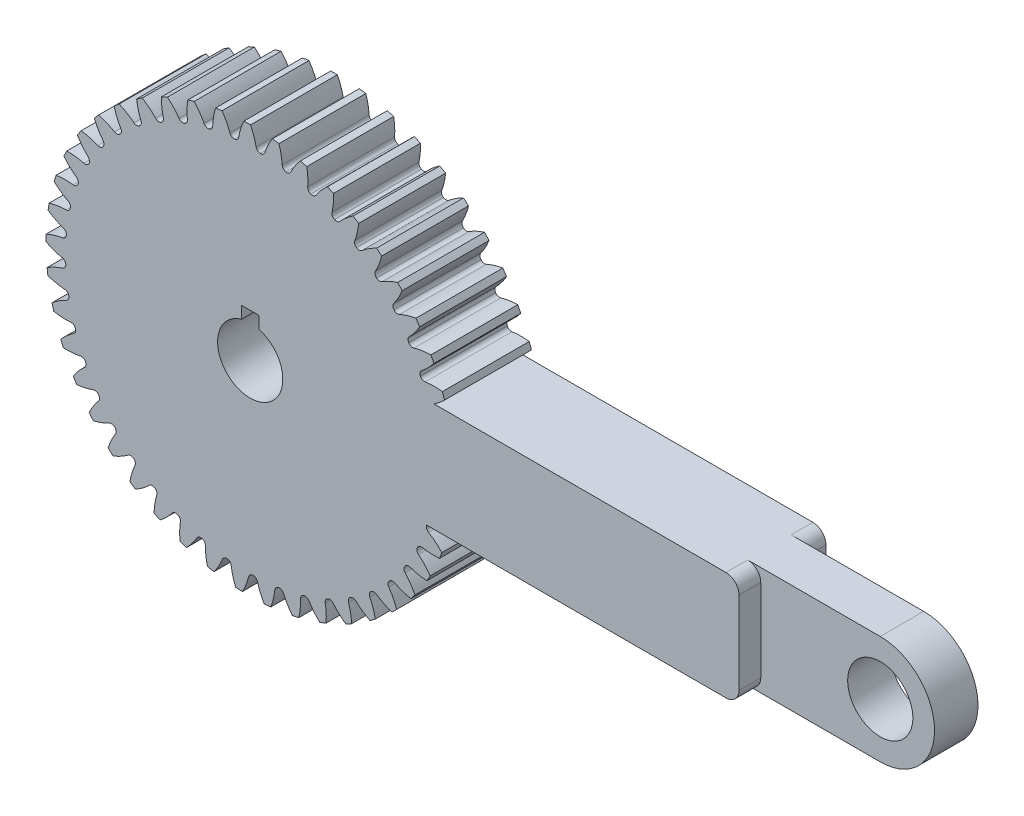
SolidWorks part; units mm, degrees
ref_plane "Front Plane" through (0, 0, 0) normal (0, 0, 1) x (1, 0, 0)
ref_plane "Top Plane" through (0, 0, 0) normal (0, 1, 0) x (1, 0, 0)
ref_plane "Right Plane" through (0, 0, 0) normal (1, 0, 0) x (0, 0, -1)
ref_plane "Plane1" through (0, 0, 0) normal (0, 0, -1) x (-1, 0, 0)
sketch "Sketch1" plane through (0, 0, 0) normal (0, 0, -1) x (-1, 0, 0)
  line L0 (-2, 7.2284) -> (-2, 10)
  line L1 (-2, 10) -> (2, 10)
  line L2 (2, 10) -> (2, 7.2284)
  line L3 (-140, -12.5) -> (-40.6202, -12.5)
  line L4 (-42.285, 12.5) -> (-140, 12.5)
  arc A0 (2, 7.2284) -> (-2, 7.2284) centre (0, 0) cw
  arc A1 (-140, 12.5) -> (-140, -12.5) centre (-140, 0) ccw
  arc A2 (-40.6202, -12.5) -> (-40.6, -12.5654) centre (0, 0) ccw
  arc A3 (-40.6, -12.5654) -> (-41.0442, -13.7206) centre (-41.5553, -12.8611) cw
  arc A4 (-44.1067, -16.2358) -> (-41.0442, -13.7206) centre (-33.1834, -26.4137) cw
  arc A5 (-44.1067, -16.2358) -> (-43.552, -17.6699) centre (0, 0) ccw
  arc A6 (-39.5941, -17.4696) -> (-43.552, -17.6699) centre (-42.3312, -2.5814) cw
  arc A7 (-39.5941, -17.4696) -> (-38.4882, -18.0253) centre (-39.3938, -18.4494) cw
  arc A8 (-38.4882, -18.0253) -> (-38.4561, -18.0936) centre (0, 0) ccw
  arc A9 (-38.4561, -18.0936) -> (-38.7352, -19.2993) centre (-39.361, -18.5193) cw
  arc A10 (-41.4178, -22.2163) -> (-38.7352, -19.2993) centre (-29.1844, -30.7749) cw
  arc A11 (-41.4178, -22.2163) -> (-40.669, -23.5592) centre (0, 0) ccw
  arc A12 (-36.7775, -22.8101) -> (-40.669, -23.5592) centre (-41.56, -8.4477) cw
  arc A13 (-36.7775, -22.8101) -> (-35.605, -23.2064) centre (-36.4428, -23.7524) cw
  arc A14 (-35.605, -23.2064) -> (-35.5637, -23.2695) centre (0, 0) ccw
  arc A15 (-35.5637, -23.2695) -> (-35.6723, -24.5024) centre (-36.4005, -23.817) cw
  arc A16 (-37.9229, -27.7643) -> (-35.6723, -24.5024) centre (-24.6174, -34.5371) cw
  arc A17 (-37.9229, -27.7643) -> (-36.9944, -28.9899) centre (0, 0) ccw
  arc A18 (-33.245, -27.7065) -> (-36.9944, -28.9899) centre (-39.9799, -14.1495) cw
  arc A19 (-33.245, -27.7065) -> (-32.0288, -27.9358) centre (-32.7824, -28.5931) cw
  arc A20 (-32.0288, -27.9358) -> (-31.9791, -27.9926) centre (0, 0) ccw
  arc A21 (-31.9791, -27.9926) -> (-31.9151, -29.2286) centre (-32.7316, -28.6512) cw
  arc A22 (-33.6898, -32.7719) -> (-31.9151, -29.2286) centre (-19.5712, -37.6271) cw
  arc A23 (-33.6898, -32.7719) -> (-32.5997, -33.8564) centre (0, 0) ccw
  arc A24 (-29.0655, -32.0637) -> (-32.5997, -33.8564) centre (-37.6216, -19.5759) cw
  arc A25 (-29.0655, -32.0637) -> (-27.8292, -32.1214) centre (-28.484, -32.8772) cw
  arc A26 (-27.8292, -32.1214) -> (-27.7721, -32.1708) centre (0, 0) ccw
  arc A27 (-27.7721, -32.1708) -> (-27.5366, -33.3858) centre (-28.4256, -32.9278) cw
  arc A28 (-28.8009, -37.1417) -> (-27.5366, -33.3858) centre (-14.144, -39.9847) cw
  arc A29 (-28.8009, -37.1417) -> (-27.5706, -38.0639) centre (0, 0) ccw
  arc A30 (-24.3202, -35.7968) -> (-27.5706, -38.0639) centre (-34.531, -24.6213) cw
  arc A31 (-24.3202, -35.7968) -> (-23.0879, -35.6819) centre (-23.6311, -36.5215) cw
  arc A32 (-23.0879, -35.6819) -> (-23.0245, -35.7228) centre (0, 0) ccw
  arc A33 (-23.0245, -35.7228) -> (-22.6223, -36.8933) centre (-23.5663, -36.5634) cw
  arc A34 (-23.3515, -40.7886) -> (-22.6223, -36.8933) centre (-8.4416, -41.564) cw
  arc A35 (-23.3515, -40.7886) -> (-22.0048, -41.5306) centre (0, 0) ccw
  arc A36 (-19.1016, -38.8331) -> (-22.0048, -41.5306) centre (-30.7683, -29.1875) cw
  arc A37 (-19.1016, -38.8331) -> (-17.8972, -38.5479) centre (-18.3184, -39.4549) cw
  arc A38 (-17.8972, -38.5479) -> (-17.8288, -38.5796) centre (0, 0) ccw
  arc A39 (-17.8288, -38.5796) -> (-17.2675, -39.6826) centre (-18.2483, -39.4873) cw
  arc A40 (-17.4476, -43.6415) -> (-17.2675, -39.6826) centre (-2.5748, -42.3343) cw
  arc A41 (-17.4476, -43.6415) -> (-16.0107, -44.1889) centre (0, 0) ccw
  arc A42 (-13.5111, -41.1136) -> (-16.0107, -44.1889) centre (-26.4068, -33.1856) cw
  arc A43 (-13.5111, -41.1136) -> (-12.3582, -40.6635) centre (-12.649, -41.6203) cw
  arc A44 (-12.3582, -40.6635) -> (-12.286, -40.6854) centre (0, 0) ccw
  arc A45 (-12.286, -40.6854) -> (-11.5767, -41.6996) centre (-12.5751, -41.6427) cw
  arc A46 (-11.2041, -45.645) -> (-11.5767, -41.6996) centre (3.342, -42.2807) cw
  arc A47 (-11.2041, -45.645) -> (-9.705, -45.9871) centre (0, 0) ccw
  arc A48 (-7.6577, -42.5939) -> (-9.705, -45.9871) centre (-21.5312, -36.5377) cw
  arc A49 (-7.6577, -42.5939) -> (-6.5787, -41.9877) centre (-6.7335, -42.9757) cw
  arc A50 (-6.5787, -41.9877) -> (-6.5042, -41.9994) centre (0, 0) ccw
  arc A51 (-6.5042, -41.9994) -> (-5.6606, -42.905) centre (-6.6572, -42.9876) cw
  arc A52 (-4.7425, -46.7601) -> (-5.6606, -42.905) centre (9.1938, -41.4041) cw
  arc A53 (-4.7425, -46.7601) -> (-3.2104, -46.8902) centre (0, 0) ccw
  arc A54 (-1.6553, -43.2451) -> (-3.2104, -46.8902) centre (-16.2366, -39.1787) cw
  arc A55 (-1.6553, -43.2451) -> (-0.6711, -42.4947) centre (-0.6869, -43.4946) cw
  arc A56 (-0.6711, -42.4947) -> (-0.5957, -42.4958) centre (0, 0) ccw
  arc A57 (-0.5957, -42.4958) -> (0.3657, -43.2752) centre (-0.6097, -43.4957) cw
  arc A58 (1.8114, -46.9651) -> (0.3657, -43.2752) centre (14.8667, -39.7216) cw
  arc A59 (1.8114, -46.9651) -> (3.3467, -46.8807) centre (0, 0) ccw
  arc A60 (4.3794, -43.0546) -> (3.3467, -46.8807) centre (-10.626, -41.0571) cw
  arc A61 (4.3794, -43.0546) -> (5.2495, -42.1745) centre (5.3731, -43.1669) cw
  arc A62 (5.2495, -42.1745) -> (5.3244, -42.1652) centre (0, 0) ccw
  arc A63 (5.3244, -42.1652) -> (6.3849, -42.8032) centre (5.4497, -43.1573) cw
  arc A64 (8.3301, -46.2559) -> (6.3849, -42.8032) centre (20.2502, -37.266) cw
  arc A65 (8.3301, -46.2559) -> (9.8387, -45.9587) centre (0, 0) ccw
  arc A66 (10.3288, -42.0261) -> (9.8387, -45.9587) centre (-4.8085, -42.1364) cw
  arc A67 (10.3288, -42.0261) -> (11.068, -41.0335) centre (11.3284, -41.999) cw
  arc A68 (11.068, -41.0335) -> (11.1408, -41.0138) centre (0, 0) ccw
  arc A69 (11.1408, -41.0138) -> (12.2798, -41.498) centre (11.403, -41.9788) cw
  arc A70 (14.6866, -44.6464) -> (12.2798, -41.498) centre (25.2395, -34.0851) cw
  arc A71 (14.6866, -44.6464) -> (16.1392, -44.1421) centre (0, 0) ccw
  arc A72 (16.0772, -40.1797) -> (16.1392, -44.1421) centre (1.1025, -42.3955) cw
  arc A73 (16.0772, -40.1797) -> (16.6711, -39.0938) centre (17.0633, -40.0137) cw
  arc A74 (16.6711, -39.0938) -> (16.7404, -39.0642) centre (0, 0) ccw
  arc A75 (16.7404, -39.0642) -> (17.9357, -39.3852) centre (17.1343, -39.9833) cw
  arc A76 (20.7573, -42.168) -> (17.9357, -39.3852) centre (29.7376, -30.2407) cw
  arc A77 (20.7573, -42.168) -> (22.1255, -41.4664) centre (0, 0) ccw
  arc A78 (21.5127, -37.5511) -> (22.1255, -41.4664) centre (6.9921, -41.8295) cw
  arc A79 (21.5127, -37.5511) -> (21.9496, -36.3932) centre (22.4661, -37.2495) cw
  arc A80 (21.9496, -36.3932) -> (22.0142, -36.3542) centre (0, 0) ccw
  arc A81 (22.0142, -36.3542) -> (23.2425, -36.5057) centre (22.5322, -37.2096) cw
  arc A82 (26.4239, -38.8687) -> (23.2425, -36.5057) centre (33.6569, -25.8077) cw
  arc A83 (26.4239, -38.8687) -> (27.6812, -37.9836) centre (0, 0) ccw
  arc A84 (26.5294, -34.1917) -> (27.6812, -37.9836) centre (12.7456, -40.4493) cw
  arc A85 (26.5294, -34.1917) -> (26.801, -32.9842) centre (27.4316, -33.7603) cw
  arc A86 (26.801, -32.9842) -> (26.8595, -32.9366) centre (0, 0) ccw
  arc A87 (26.8595, -32.9366) -> (28.0969, -32.9157) centre (27.4915, -33.7116) cw
  arc A88 (31.5762, -34.813) -> (28.0969, -32.9157) centre (36.9211, -20.8724) cw
  arc A89 (31.5762, -34.813) -> (32.6981, -33.7615) centre (0, 0) ccw
  arc A90 (31.0298, -30.1668) -> (32.6981, -33.7615) centre (18.251, -38.2818) cw
  arc A91 (31.0298, -30.1668) -> (31.1307, -28.9332) centre (31.8631, -29.614) cw
  arc A92 (31.1307, -28.9332) -> (31.182, -28.8779) centre (0, 0) ccw
  arc A93 (31.182, -28.8779) -> (32.4045, -28.685) centre (31.9157, -29.5574) cw
  arc A94 (36.114, -30.0796) -> (32.4045, -28.685) centre (39.4667, -15.5309) cw
  arc A95 (36.114, -30.0796) -> (37.0785, -28.8822) centre (0, 0) ccw
  arc A96 (34.9262, -25.5547) -> (37.0785, -28.8822) centre (23.4012, -35.3692) cw
  arc A97 (34.9262, -25.5547) -> (34.8544, -24.3191) centre (35.6745, -24.8913) cw
  arc A98 (34.8544, -24.3191) -> (34.8975, -24.2572) centre (0, 0) ccw
  arc A99 (34.8975, -24.2572) -> (36.0813, -23.896) centre (35.7187, -24.828) cw
  arc A100 (39.9488, -24.7608) -> (36.0813, -23.896) centre (41.2441, -9.887) cw
  arc A101 (39.9488, -24.7608) -> (40.7373, -23.4408) centre (0, 0) ccw
  arc A102 (38.1428, -20.4452) -> (40.7373, -23.4408) centre (28.0959, -31.7682) cw
  arc A103 (38.1428, -20.4452) -> (37.8998, -19.2316) centre (38.7915, -19.6842) cw
  arc A104 (37.8998, -19.2316) -> (37.9339, -19.1643) centre (0, 0) ccw
  arc A105 (37.9339, -19.1643) -> (39.0558, -18.6419) centre (38.8264, -19.6153) cw
  arc A106 (43.006, -18.96) -> (39.0558, -18.6419) centre (42.2187, -4.0507) cw
  arc A107 (43.006, -18.96) -> (43.6032, -17.5431) centre (0, 0) ccw
  arc A108 (40.617, -14.9378) -> (43.6032, -17.5431) centre (32.2438, -27.5488) cw
  arc A109 (40.617, -14.9378) -> (40.2075, -13.7699) centre (41.1535, -14.0939) cw
  arc A110 (40.2075, -13.7699) -> (40.2319, -13.6985) centre (0, 0) ccw
  arc A111 (40.2319, -13.6985) -> (41.2702, -13.025) centre (41.1785, -14.0208) cw
  arc A112 (45.2262, -12.7902) -> (41.2702, -13.025) centre (42.3716, 1.8644) cw
  arc A113 (45.2262, -12.7902) -> (45.6204, -11.304) centre (0, 0) ccw
  arc A114 (42.3007, -9.1396) -> (45.6204, -11.304) centre (35.764, -22.7933) cw
  arc A115 (42.3007, -9.1396) -> (41.7326, -8.04) centre (42.7145, -8.2292) cw
  arc A116 (41.7326, -8.04) -> (41.7468, -7.9659) centre (0, 0) ccw
  arc A117 (41.7468, -7.9659) -> (42.6813, -7.1545) centre (42.7291, -8.1534) cw
  arc A118 (46.5661, -6.3715) -> (42.6813, -7.1545) centre (41.6997, 7.7432) cw
  arc A119 (46.5661, -6.3715) -> (46.7496, -4.8449) centre (0, 0) ccw
  arc A120 (43.161, -3.1635) -> (46.7496, -4.8449) centre (38.5882, -17.5941) cw
  arc A121 (43.161, -3.1635) -> (42.4454, -2.1538) centre (43.4441, -2.2044) cw
  arc A122 (42.4454, -2.1538) -> (42.4491, -2.0784) centre (0, 0) ccw
  arc A123 (42.4491, -2.0784) -> (43.2616, -1.1448) centre (43.448, -2.1273) cw
  arc A124 (46.9997, 0.1713) -> (43.2616, -1.1448) centre (40.2163, 13.4714) cw
  arc A125 (46.9997, 0.1713) -> (46.9689, 1.7086) centre (0, 0) ccw
  arc A126 (43.1812, 2.8741) -> (46.9689, 1.7086) centre (40.6613, -12.0524) cw
  arc A127 (43.1812, 2.8741) -> (42.3321, 3.7745) centre (43.3281, 3.8633) cw
  arc A128 (42.3321, 3.7745) -> (42.3253, 3.8496) centre (0, 0) ccw
  arc A129 (42.3253, 3.8496) -> (43, 4.8872) centre (43.3212, 3.9402) cw
  arc A130 (46.5185, 6.7107) -> (43, 4.8872) centre (37.95, 18.9373) cw
  arc A131 (46.5185, 6.7107) -> (46.274, 8.2288) centre (0, 0) ccw
  arc A132 (42.361, 8.8558) -> (46.274, 8.2288) centre (41.9429, -6.2762) cw
  arc A133 (42.361, 8.8558) -> (41.3948, 9.6292) centre (42.3688, 9.8558) cw
  arc A134 (41.3948, 9.6292) -> (41.3776, 9.7027) centre (0, 0) ccw
  arc A135 (41.3776, 9.7027) -> (41.9013, 10.8241) centre (42.3512, 9.931) cw
  arc A136 (45.1318, 13.1195) -> (41.9013, 10.8241) centre (34.9451, 24.0346) cw
  arc A137 (45.1318, 13.1195) -> (44.6785, 14.5888) centre (0, 0) ccw
  arc A138 (40.7163, 14.6651) -> (44.6785, 14.5888) centre (42.4082, -0.3777) cw
  arc A139 (40.7163, 14.6651) -> (39.6518, 15.2965) centre (40.5848, 15.6565) cw
  arc A140 (39.6518, 15.2965) -> (39.6246, 15.3669) centre (0, 0) ccw
  arc A141 (39.6246, 15.3669) -> (39.9871, 16.5503) centre (40.5569, 15.7285) cw
  arc A142 (42.8667, 19.273) -> (39.9871, 16.5503) centre (31.2601, 28.6641) cw
  arc A143 (42.8667, 19.273) -> (42.2133, 20.6649) centre (0, 0) ccw
  arc A144 (38.279, 20.189) -> (42.2133, 20.6649) centre (42.0481, 5.528) cw
  arc A145 (38.279, 20.189) -> (37.137, 20.6661) centre (38.0109, 21.1524) cw
  arc A146 (37.137, 20.6661) -> (37.1003, 20.732) centre (0, 0) ccw
  arc A147 (37.1003, 20.732) -> (37.2946, 21.9543) centre (37.9733, 21.2199) cw
  arc A148 (39.7672, 25.0513) -> (37.2946, 21.9543) centre (26.9666, 32.7357) cw
  arc A149 (39.7672, 25.0513) -> (38.9265, 26.3387) centre (0, 0) ccw
  arc A150 (35.0967, 25.32) -> (38.9265, 26.3387) centre (40.8695, 11.3262) cw
  arc A151 (35.0967, 25.32) -> (33.8995, 25.6335) centre (34.6971, 26.2366) cw
  arc A152 (33.8995, 25.6335) -> (33.8539, 25.6936) centre (0, 0) ccw
  arc A153 (33.8539, 25.6936) -> (33.8762, 26.9311) centre (34.6505, 26.2982) cw
  arc A154 (35.8937, 30.342) -> (33.8762, 26.9311) centre (22.1482, 36.1702) cw
  arc A155 (35.8937, 30.342) -> (34.882, 31.4999) centre (0, 0) ccw
  arc A156 (31.2313, 29.9581) -> (34.882, 31.4999) centre (38.8955, 16.9039) cw
  arc A157 (31.2313, 29.9581) -> (30.0021, 30.1019) centre (30.708, 30.8102) cw
  arc A158 (30.0021, 30.1019) -> (29.9486, 30.1551) centre (0, 0) ccw
  arc A159 (29.9486, 30.1551) -> (29.7984, 31.3836) centre (30.6532, 30.8647) cw
  arc A160 (31.3216, 35.0422) -> (29.7984, 31.3836) centre (16.8988, 38.9006) cw
  arc A161 (31.3216, 35.0422) -> (30.1586, 36.048) centre (0, 0) ccw
  arc A162 (26.758, 34.0131) -> (30.1586, 36.048) centre (36.1644, 22.1526) cw
  arc A163 (26.758, 34.0131) -> (25.5207, 33.9845) centre (26.1212, 34.7841) cw
  arc A164 (25.5207, 33.9845) -> (25.4603, 34.0297) centre (0, 0) ccw
  arc A165 (25.4603, 34.0297) -> (25.1407, 35.2254) centre (26.0594, 34.8304) cw
  arc A166 (26.1399, 39.0603) -> (25.1407, 35.2254) centre (11.3204, 40.8739) cw
  arc A167 (26.1399, 39.0603) -> (24.8482, 39.8944) centre (0, 0) ccw
  arc A168 (21.7639, 37.4061) -> (24.8482, 39.8944) centre (32.7294, 26.9701) cw
  arc A169 (21.7639, 37.4061) -> (20.5426, 37.2055) centre (21.026, 38.0809) cw
  arc A170 (20.5426, 37.2055) -> (20.4765, 37.2419) centre (0, 0) ccw
  arc A171 (20.4765, 37.2419) -> (19.9936, 38.3815) centre (20.9583, 38.1182) cw
  arc A172 (20.4494, 42.3181) -> (19.9936, 38.3815) centre (5.5217, 42.0516) cw
  arc A173 (20.4494, 42.3181) -> (19.0542, 42.9644) centre (0, 0) ccw
  arc A174 (16.3462, 40.071) -> (19.0542, 42.9644) centre (28.6573, 31.2627) cw
  arc A175 (16.3462, 40.071) -> (15.1647, 39.7024) centre (15.5215, 40.6366) cw
  arc A176 (15.1647, 39.7024) -> (15.0942, 39.7293) centre (0, 0) ccw
  arc A177 (15.0942, 39.7293) -> (14.4574, 40.7905) centre (15.4493, 40.6641) cw
  arc A178 (14.3608, 44.7523) -> (14.4574, 40.7905) centre (-0.3845, 42.4108) cw
  arc A179 (14.3608, 44.7523) -> (12.8892, 45.1981) centre (0, 0) ccw
  arc A180 (10.6103, 41.956) -> (12.8892, 45.1981) centre (24.0275, 34.9468) cw
  arc A181 (10.6103, 41.956) -> (9.4916, 41.4266) centre (9.7149, 42.4013) cw
  arc A182 (9.4916, 41.4266) -> (9.418, 41.4433) centre (0, 0) ccw
  arc A183 (9.418, 41.4433) -> (8.6397, 42.4056) centre (9.6396, 42.4185) cw
  arc A184 (7.9927, 46.3154) -> (8.6397, 42.4056) centre (-6.2832, 41.9446) cw
  arc A185 (7.9927, 46.3154) -> (6.4734, 46.5521) centre (0, 0) ccw
  arc A186 (4.6679, 43.0243) -> (6.4734, 46.5521) centre (18.93, 37.9506) cw
  arc A187 (4.6679, 43.0243) -> (3.6338, 42.3444) centre (3.7193, 43.3407) cw
  arc A188 (3.6338, 42.3444) -> (3.5586, 42.3508) centre (0, 0) ccw
  arc A189 (3.5586, 42.3508) -> (2.6539, 43.1953) centre (3.6423, 43.3472) cw
  arc A190 (1.4691, 46.977) -> (2.6539, 43.1953) centre (-12.0596, 40.6619) cw
  arc A191 (1.4691, 46.977) -> (-0.0683, 47) centre (0, 0) ccw
  arc A192 (-1.3654, 43.2552) -> (-0.0683, 47) centre (13.4641, 40.2159) cw
  arc A193 (-1.3654, 43.2552) -> (-2.2948, 42.438) centre (-2.3488, 43.4365) cw
  arc A194 (-2.2948, 42.438) -> (-2.3701, 42.4339) centre (0, 0) ccw
  arc A195 (-2.3701, 42.4339) -> (-3.3835, 43.1443) centre (-2.4259, 43.4323) cw
  arc A196 (-5.0832, 46.7243) -> (-3.3835, 43.1443) centre (-17.6013, 38.5878) cw
  arc A197 (-5.0832, 46.7243) -> (-6.6088, 46.533) centre (0, 0) ccw
  arc A198 (-7.372, 42.6443) -> (-6.6088, 46.533) centre (7.7361, 41.6983) cw
  arc A199 (-7.372, 42.6443) -> (-8.1787, 41.7056) centre (-8.3711, 42.6869) cw
  arc A200 (-8.1787, 41.7056) -> (-8.2527, 41.691) centre (0, 0) ccw
  arc A201 (-8.2527, 41.691) -> (-9.3551, 42.2535) centre (-8.4469, 42.672) cw
  arc A202 (-11.5365, 45.5622) -> (-9.3551, 42.2535) centre (-22.8004, 35.7627) cw
  arc A203 (-11.5365, 45.5622) -> (-13.0206, 45.1604) centre (0, 0) ccw
  arc A204 (-13.2352, 41.2033) -> (-13.0206, 45.1604) centre (1.8575, 42.3692) cw
  arc A205 (-13.2352, 41.2033) -> (-13.9034, 40.1615) centre (-14.2305, 41.1065) cw
  arc A206 (-13.9034, 40.1615) -> (-13.9747, 40.1367) centre (0, 0) ccw
  arc A207 (-13.9747, 40.1367) -> (-15.1446, 40.5404) centre (-14.3035, 41.0811) cw
  arc A208 (-17.7652, 43.5132) -> (-15.1446, 40.5404) centre (-27.5557, 32.2414) cw
  arc A209 (-17.7652, 43.5132) -> (-19.179, 42.9088) centre (0, 0) ccw
  arc A210 (-18.8408, 38.9603) -> (-19.179, 42.9088) centre (-4.0572, 42.2154) cw
  arc A211 (-18.8408, 38.9603) -> (-19.3575, 37.8357) centre (-19.813, 38.7259) cw
  arc A212 (-19.3575, 37.8357) -> (-19.4246, 37.8012) centre (0, 0) ccw
  arc A213 (-19.4246, 37.8012) -> (-20.6394, 38.0381) centre (-19.8817, 38.6907) cw
  arc A214 (-23.6482, 40.6173) -> (-20.6394, 38.0381) centre (-31.7747, 28.0926) cw
  arc A215 (-23.6482, 40.6173) -> (-24.9641, 39.822) centre (0, 0) ccw
  arc A216 (-24.0797, 35.959) -> (-24.9641, 39.822) centre (-9.8929, 41.2399) cw
  arc A217 (-24.0797, 35.959) -> (-24.4348, 34.7734) centre (-25.0098, 35.5916) cw
  arc A218 (-24.4348, 34.7734) -> (-24.4965, 34.73) centre (0, 0) ccw
  arc A219 (-24.4965, 34.73) -> (-25.7324, 34.7955) centre (-25.0729, 35.5472) cw
  arc A220 (-29.0709, 36.9308) -> (-25.7324, 34.7955) centre (-35.3752, 23.397) cw
  arc A221 (-29.0709, 36.9308) -> (-30.2633, 35.9601) centre (0, 0) ccw
  arc A222 (-28.8499, 32.2578) -> (-30.2633, 35.9601) centre (-15.5361, 39.4617) cw
  arc A223 (-28.8499, 32.2578) -> (-29.0365, 31.0343) centre (-29.7198, 31.7645) cw
  arc A224 (-29.0365, 31.0343) -> (-29.0916, 30.9827) centre (0, 0) ccw
  arc A225 (-29.0916, 30.9827) -> (-30.3246, 30.8756) centre (-29.7761, 31.7117) cw
  arc A226 (-33.9277, 32.5255) -> (-30.3246, 30.8756) centre (-38.2872, 18.2461) cw
  arc A227 (-33.9277, 32.5255) -> (-34.9735, 31.3983) centre (0, 0) ccw
  arc A228 (-33.0585, 27.9287) -> (-34.9735, 31.3983) centre (-20.877, 36.9154) cw
  arc A229 (-33.0585, 27.9287) -> (-33.0731, 26.6912) centre (-33.8513, 27.3192) cw
  arc A230 (-33.0731, 26.6912) -> (-33.1204, 26.6324) centre (0, 0) ccw
  arc A231 (-33.1204, 26.6324) -> (-34.3265, 26.3547) centre (-33.8997, 27.2591) cw
  arc A232 (-38.1242, 27.4871) -> (-34.3265, 26.3547) centre (-40.4539, 12.74) cw
  arc A233 (-38.1242, 27.4871) -> (-39.0029, 26.2254) centre (0, 0) ccw
  arc A234 (-36.6237, 23.0561) -> (-39.0029, 26.2254) centre (-25.8114, 33.6507) cw
  arc A235 (-36.6237, 23.0561) -> (-36.4659, 21.8286) centre (-37.324, 22.3422) cw
  arc A236 (-36.4659, 21.8286) -> (-36.5046, 21.7638) centre (0, 0) ccw
  arc A237 (-36.5046, 21.7638) -> (-37.6603, 21.3209) centre (-37.3636, 22.2759) cw
  arc A238 (-41.5787, 21.9138) -> (-37.6603, 21.3209) centre (-41.8333, 6.9859) cw
  arc A239 (-41.5787, 21.9138) -> (-42.2732, 20.542) centre (0, 0) ccw
  arc A240 (-39.4761, 17.7347) -> (-42.2732, 20.542) centre (-30.2435, 29.7309) cw
  arc A241 (-39.4761, 17.7347) -> (-39.149, 16.541) centre (-40.0701, 16.9302) cw
  arc A242 (-39.149, 16.541) -> (-39.1783, 16.4715) centre (0, 0) ccw
  arc A243 (-39.1783, 16.4715) -> (-40.2611, 15.8721) centre (-40.1001, 16.8591) cw
  arc A244 (-44.2238, 15.9139) -> (-40.2611, 15.8721) centre (-42.3984, 1.0958) cw
  arc A245 (-44.2238, 15.9139) -> (-44.7207, 14.4588) centre (0, 0) ccw
  arc A246 (-42.285, 12.5) -> (-44.7207, 14.4588) centre (-33.0921, 26.4253) cw
  circle A247 centre (-140, 0) radius 7.5
  dimension "D1" = 15
  dimension "D2" = 7.5
  dimension "D3" = 12.5
  dimension "D4" = 42.5
  dimension "D5" = 1
  dimension "D6" = 14.9301
  dimension "D7" = 47
  dimension "D8" = 15.1377
  dimension "D9" = 1
  dimension "D10" = 42.5
  dimension "D11" = 1
  dimension "D12" = 14.9301
  dimension "D13" = 47
  dimension "D14" = 15.1377
  dimension "D15" = 1
  dimension "D16" = 42.5
  dimension "D17" = 1
  dimension "D18" = 14.9301
  dimension "D19" = 47
  dimension "D20" = 15.1377
  dimension "D21" = 1
  dimension "D22" = 42.5
  dimension "D23" = 1
  dimension "D24" = 14.9301
  dimension "D25" = 47
  dimension "D26" = 15.1377
  dimension "D27" = 1
  dimension "D28" = 42.5
  dimension "D29" = 1
  dimension "D30" = 14.9301
  dimension "D31" = 47
  dimension "D32" = 15.1377
  dimension "D33" = 1
  dimension "D34" = 42.5
  dimension "D35" = 1
  dimension "D36" = 14.9301
  dimension "D37" = 47
  dimension "D38" = 15.1377
  dimension "D39" = 1
  dimension "D40" = 42.5
  dimension "D41" = 1
  dimension "D42" = 14.9301
  dimension "D43" = 47
  dimension "D44" = 15.1377
  dimension "D45" = 1
  dimension "D46" = 42.5
  dimension "D47" = 1
  dimension "D48" = 14.9301
  dimension "D49" = 47
  dimension "D50" = 15.1377
  dimension "D51" = 1
  dimension "D52" = 42.5
  dimension "D53" = 1
  dimension "D54" = 14.9301
  dimension "D55" = 47
  dimension "D56" = 15.1377
  dimension "D57" = 1
  dimension "D58" = 42.5
  dimension "D59" = 1
  dimension "D60" = 14.9301
  dimension "D61" = 47
  dimension "D62" = 15.1377
  dimension "D63" = 1
  dimension "D64" = 42.5
  dimension "D65" = 1
  dimension "D66" = 14.9301
  dimension "D67" = 47
  dimension "D68" = 15.1377
  dimension "D69" = 1
  dimension "D70" = 42.5
  dimension "D71" = 1
  dimension "D72" = 14.9301
  dimension "D73" = 47
  dimension "D74" = 15.1377
  dimension "D75" = 1
  dimension "D76" = 42.5
  dimension "D77" = 1
  dimension "D78" = 14.9301
  dimension "D79" = 47
  dimension "D80" = 15.1377
  dimension "D81" = 1
  dimension "D82" = 42.5
  dimension "D83" = 1
  dimension "D84" = 14.9301
  dimension "D85" = 47
  dimension "D86" = 15.1377
  dimension "D87" = 1
  dimension "D88" = 42.5
  dimension "D89" = 1
  dimension "D90" = 14.9301
  dimension "D91" = 47
  dimension "D92" = 15.1377
  dimension "D93" = 1
  dimension "D94" = 42.5
  dimension "D95" = 1
  dimension "D96" = 14.9301
  dimension "D97" = 47
  dimension "D98" = 15.1377
  dimension "D99" = 1
  dimension "D100" = 42.5
  dimension "D101" = 1
  dimension "D102" = 14.9301
  dimension "D103" = 47
  dimension "D104" = 15.1377
  dimension "D105" = 1
  dimension "D106" = 42.5
  dimension "D107" = 1
  dimension "D108" = 14.9301
  dimension "D109" = 47
  dimension "D110" = 15.1377
  dimension "D111" = 1
  dimension "D112" = 42.5
  dimension "D113" = 1
  dimension "D114" = 14.9301
  dimension "D115" = 47
  dimension "D116" = 15.1377
  dimension "D117" = 1
  dimension "D118" = 42.5
  dimension "D119" = 1
  dimension "D120" = 14.9301
  dimension "D121" = 47
  dimension "D122" = 15.1377
  dimension "D123" = 1
  dimension "D124" = 42.5
  dimension "D125" = 1
  dimension "D126" = 14.9301
  dimension "D127" = 47
  dimension "D128" = 15.1377
  dimension "D129" = 1
  dimension "D130" = 42.5
  dimension "D131" = 1
  dimension "D132" = 14.9301
  dimension "D133" = 47
  dimension "D134" = 15.1377
  dimension "D135" = 1
  dimension "D136" = 42.5
  dimension "D137" = 1
  dimension "D138" = 14.9301
  dimension "D139" = 47
  dimension "D140" = 15.1377
  dimension "D141" = 1
  dimension "D142" = 42.5
  dimension "D143" = 1
  dimension "D144" = 14.9301
  dimension "D145" = 47
  dimension "D146" = 15.1377
  dimension "D147" = 1
  dimension "D148" = 42.5
  dimension "D149" = 1
  dimension "D150" = 14.9301
  dimension "D151" = 47
  dimension "D152" = 15.1377
  dimension "D153" = 1
  dimension "D154" = 42.5
  dimension "D155" = 1
  dimension "D156" = 14.9301
  dimension "D157" = 47
  dimension "D158" = 15.1377
  dimension "D159" = 1
  dimension "D160" = 42.5
  dimension "D161" = 1
  dimension "D162" = 14.9301
  dimension "D163" = 47
  dimension "D164" = 15.1377
  dimension "D165" = 1
  dimension "D166" = 42.5
  dimension "D167" = 1
  dimension "D168" = 14.9301
  dimension "D169" = 47
  dimension "D170" = 15.1377
  dimension "D171" = 1
  dimension "D172" = 42.5
  dimension "D173" = 1
  dimension "D174" = 14.9301
  dimension "D175" = 47
  dimension "D176" = 15.1377
  dimension "D177" = 1
  dimension "D178" = 42.5
  dimension "D179" = 1
  dimension "D180" = 14.9301
  dimension "D181" = 47
  dimension "D182" = 15.1377
  dimension "D183" = 1
  dimension "D184" = 42.5
  dimension "D185" = 1
  dimension "D186" = 14.9301
  dimension "D187" = 47
  dimension "D188" = 15.1377
  dimension "D189" = 1
  dimension "D190" = 42.5
  dimension "D191" = 1
  dimension "D192" = 14.9301
  dimension "D193" = 47
  dimension "D194" = 15.1377
  dimension "D195" = 1
  dimension "D196" = 42.5
  dimension "D197" = 1
  dimension "D198" = 14.9301
  dimension "D199" = 47
  dimension "D200" = 15.1377
  dimension "D201" = 1
  dimension "D202" = 42.5
  dimension "D203" = 1
  dimension "D204" = 14.9301
  dimension "D205" = 47
  dimension "D206" = 15.1377
  dimension "D207" = 1
  dimension "D208" = 42.5
  dimension "D209" = 1
  dimension "D210" = 14.9301
  dimension "D211" = 47
  dimension "D212" = 15.1377
  dimension "D213" = 1
  dimension "D214" = 42.5
  dimension "D215" = 1
  dimension "D216" = 14.9301
  dimension "D217" = 47
  dimension "D218" = 15.1377
  dimension "D219" = 1
  dimension "D220" = 42.5
  dimension "D221" = 1
  dimension "D222" = 14.9301
  dimension "D223" = 47
  dimension "D224" = 15.1377
  dimension "D225" = 1
  dimension "D226" = 42.5
  dimension "D227" = 1
  dimension "D228" = 14.9301
  dimension "D229" = 47
  dimension "D230" = 15.1377
  dimension "D231" = 1
  dimension "D232" = 42.5
  dimension "D233" = 1
  dimension "D234" = 14.9301
  dimension "D235" = 47
  dimension "D236" = 15.1377
  dimension "D237" = 1
  dimension "D238" = 42.5
  dimension "D239" = 1
  dimension "D240" = 14.9301
  dimension "D241" = 47
  dimension "D242" = 15.1377
  dimension "D243" = 1
  dimension "D244" = 42.5
  dimension "D245" = 1
  dimension "D246" = 14.9301
  dimension "D247" = 47
  dimension "D248" = 16.686
  dimension "D249" = 0.3447
  dimension "D250" = 0.6346
  dimension "D251" = 1.3131
  dimension "D252" = 1.3289
  dimension "D253" = 1.3903
  dimension "D254" = 1.6155
  dimension "D255" = 1.9317
  dimension "D256" = 2.3657
  dimension "D257" = 3.1025
  dimension "D258" = 3.4691
  dimension "D259" = 3.8114
  dimension "D260" = 3.8575
  dimension "D261" = 4.6539
  dimension "D262" = 5.342
  dimension "D263" = 5.3467
  dimension "D264" = 5.5586
  dimension "D265" = 5.6338
  dimension "D266" = 6.3794
  dimension "D267" = 6.6679
  dimension "D268" = 7.2495
  dimension "D269" = 7.3244
  dimension "D270" = 7.5217
  dimension "D271" = 8.3849
  dimension "D272" = 8.4734
  dimension "D273" = 8.9921
  dimension "D274" = 9.7361
  dimension "D275" = 9.9927
  dimension "D276" = 10.3301
  dimension "D277" = 10.6397
  dimension "D278" = 11.1938
  dimension "D279" = 11.418
  dimension "D280" = 11.4916
  dimension "D281" = 11.8387
  dimension "D282" = 12.3288
  dimension "D283" = 12.6103
  dimension "D284" = 13.068
  dimension "D285" = 13.1408
  dimension "D286" = 13.3204
  dimension "D287" = 14.2798
  dimension "D288" = 14.7456
  dimension "D289" = 14.8892
  dimension "D290" = 15.4641
  dimension "D291" = 16.3608
  dimension "D292" = 16.4574
  dimension "D293" = 16.6866
  dimension "D294" = 17.1647
  dimension "D295" = 18.0772
  dimension "D296" = 18.1392
  dimension "D297" = 18.3462
  dimension "D298" = 18.7404
  dimension "D299" = 18.8988
  dimension "D300" = 19.9357
  dimension "D301" = 20.251
  dimension "D302" = 21.0542
  dimension "D303" = 21.9936
  dimension "D304" = 22.4494
  dimension "D305" = 22.5426
  dimension "D306" = 22.7573
  dimension "D307" = 23.5127
  dimension "D308" = 23.7639
  dimension "D309" = 23.9496
  dimension "D310" = 24.0142
  dimension "D311" = 24.1482
  dimension "D312" = 25.2425
  dimension "D313" = 25.4012
  dimension "D314" = 26.8482
  dimension "D315" = 27.1407
  dimension "D316" = 27.4603
  dimension "D317" = 27.5207
  dimension "D318" = 28.4239
  dimension "D319" = 28.5294
  dimension "D320" = 28.758
  dimension "D321" = 28.801
  dimension "D322" = 28.8595
  dimension "D323" = 28.9666
  dimension "D324" = 30.0959
  dimension "D325" = 30.0969
  dimension "D326" = 31.7984
  dimension "D327" = 31.9486
  dimension "D328" = 32.0021
  dimension "D329" = 32.1586
  dimension "D330" = 33.0298
  dimension "D331" = 33.1307
  dimension "D332" = 33.182
  dimension "D333" = 33.2313
  dimension "D334" = 33.2601
  dimension "D335" = 33.5762
  dimension "D336" = 34.2438
  dimension "D337" = 34.4045
  dimension "D338" = 35.8539
  dimension "D339" = 35.8762
  dimension "D340" = 35.8995
  dimension "D341" = 36.8544
  dimension "D342" = 36.882
  dimension "D343" = 36.8975
  dimension "D344" = 36.9262
  dimension "D345" = 36.9451
  dimension "D346" = 37.0967
  dimension "D347" = 37.764
  dimension "D348" = 38.0813
  dimension "D349" = 38.114
  dimension "D350" = 39.1003
  dimension "D351" = 39.137
  dimension "D352" = 39.2946
  dimension "D353" = 39.8998
  dimension "D354" = 39.9339
  dimension "D355" = 39.95
  dimension "D356" = 40.1428
  dimension "D357" = 40.279
  dimension "D358" = 40.5882
  dimension "D359" = 40.9265
  dimension "D360" = 41.0558
  dimension "D361" = 41.6246
  dimension "D362" = 41.6518
  dimension "D363" = 41.9488
  dimension "D364" = 41.9871
  dimension "D365" = 42.2075
  dimension "D366" = 42.2163
  dimension "D367" = 42.2319
  dimension "D368" = 42.617
  dimension "D369" = 42.6613
  dimension "D370" = 42.7163
  dimension "D371" = 43.2702
  dimension "D372" = 43.3776
  dimension "D373" = 43.3948
  dimension "D374" = 43.6997
  dimension "D375" = 43.7326
  dimension "D376" = 43.7468
  dimension "D377" = 43.9013
  dimension "D378" = 43.9429
  dimension "D379" = 44.0481
  dimension "D380" = 44.2187
  dimension "D381" = 44.3007
  dimension "D382" = 44.3253
  dimension "D383" = 44.3321
  dimension "D384" = 44.361
  dimension "D385" = 44.3716
  dimension "D386" = 44.4082
  dimension "D387" = 44.4454
  dimension "D388" = 44.4491
  dimension "D389" = 44.6813
  dimension "D390" = 45
  dimension "D391" = 45.161
  dimension "D392" = 45.1812
  dimension "D393" = 45.2616
  dimension "D394" = 0.3701
  dimension "D395" = 0.5748
  dimension "D396" = 1.2104
  dimension "D397" = 1.3835
  dimension "D398" = 2.0572
  dimension "D399" = 2.7425
  dimension "D400" = 3.0832
  dimension "D401" = 3.6606
  dimension "D402" = 4.5787
  dimension "D403" = 4.6088
  dimension "D404" = 5.372
  dimension "D405" = 5.6577
  dimension "D406" = 6.2527
  dimension "D407" = 6.4416
  dimension "D408" = 7.3551
  dimension "D409" = 7.705
  dimension "D410" = 7.8929
  dimension "D411" = 9.2041
  dimension "D412" = 9.5365
  dimension "D413" = 9.5767
  dimension "D414" = 10.3582
  dimension "D415" = 11.0206
  dimension "D416" = 11.2352
  dimension "D417" = 11.5111
  dimension "D418" = 11.9747
  dimension "D419" = 12.144
  dimension "D420" = 13.1446
  dimension "D421" = 13.5361
  dimension "D422" = 14.0107
  dimension "D423" = 15.2675
  dimension "D424" = 15.4476
  dimension "D425" = 15.7652
  dimension "D426" = 15.8972
  dimension "D427" = 16.8408
  dimension "D428" = 17.1016
  dimension "D429" = 17.179
  dimension "D430" = 17.4246
  dimension "D431" = 17.5712
  dimension "D432" = 18.6394
  dimension "D433" = 18.877
  dimension "D434" = 20.0048
  dimension "D435" = 20.6223
  dimension "D436" = 21.0245
  dimension "D437" = 21.0879
  dimension "D438" = 21.6482
  dimension "D439" = 22.0797
  dimension "D440" = 22.3202
  dimension "D441" = 22.4348
  dimension "D442" = 22.4965
  dimension "D443" = 22.6174
  dimension "D444" = 23.7324
  dimension "D445" = 23.8114
  dimension "D446" = 25.5366
  dimension "D447" = 25.5706
  dimension "D448" = 25.7721
  dimension "D449" = 25.8292
  dimension "D450" = 26.8499
  dimension "D451" = 27.0365
  dimension "D452" = 27.0655
  dimension "D453" = 27.0709
  dimension "D454" = 27.0916
  dimension "D455" = 27.1844
  dimension "D456" = 28.2435
  dimension "D457" = 28.3246
  dimension "D458" = 29.9151
  dimension "D459" = 29.9791
  dimension "D460" = 30.0288
  dimension "D461" = 30.5997
  dimension "D462" = 31.0585
  dimension "D463" = 31.0731
  dimension "D464" = 31.0921
  dimension "D465" = 31.1204
  dimension "D466" = 31.1834
  dimension "D467" = 31.245
  dimension "D468" = 31.9277
  dimension "D469" = 32.3265
  dimension "D470" = 33.5637
  dimension "D471" = 33.605
  dimension "D472" = 33.6723
  dimension "D473" = 34.4659
  dimension "D474" = 34.5046
  dimension "D475" = 34.6237
  dimension "D476" = 34.7775
  dimension "D477" = 34.9944
  dimension "D478" = 35.6603
  dimension "D479" = 36.1242
  dimension "D480" = 36.4561
  dimension "D481" = 36.4882
  dimension "D482" = 36.7352
  dimension "D483" = 37.149
  dimension "D484" = 37.1783
  dimension "D485" = 37.4761
  dimension "D486" = 37.5941
  dimension "D487" = 38.2611
  dimension "D488" = 38.6
  dimension "D489" = 38.669
  dimension "D490" = 39.0442
  dimension "D491" = 39.5787
  dimension "D492" = 40.285
  dimension "D493" = 40.3312
  dimension "D494" = 40.3984
  dimension "D495" = 2.5
  dimension "D660" = 138
extrude "Boss-Extrude1" add sketch "Sketch1" against normal blind 20
sketch "Sketch2" plane through (0, -12.5, 0) normal (0, -1, 0) x (1, 0, 0)
  line L0 (152.5, 0) -> (152.5, 20) construction
  line L1 (152.5, 15) -> (112.5, 15)
  line L2 (152.5, 15) -> (152.5, 22.7469)
  line L3 (152.5, 22.7469) -> (112.5, 22.7469)
  line L4 (112.5, 15) -> (112.5, 22.7469)
  line L5 (140, 0) -> (40.6202, 0) construction
  line L6 (112.5, 0) -> (152.5, 0)
  line L7 (112.5, 0) -> (112.5, 5)
  line L8 (112.5, 5) -> (152.5, 5)
  line L9 (152.5, 0) -> (152.5, 5)
  line L10 (152.5, 10) -> (100.5754, 10) construction
  dimension "D1" = 10
  dimension "D2" = 5
  dimension "D3" = 40
extrude "Cut-Extrude1" cut sketch "Sketch2" against normal blind 41
fillet "Fillet1" radius 3 4 edges at (112.5, 12.5, 2.5) (112.5, 12.5, 17.5) (112.5, -12.5, 17.5) (112.5, -12.5, 2.5)
scale "Scale1" scale about origin uniform scaling yes scale factor 0.3
